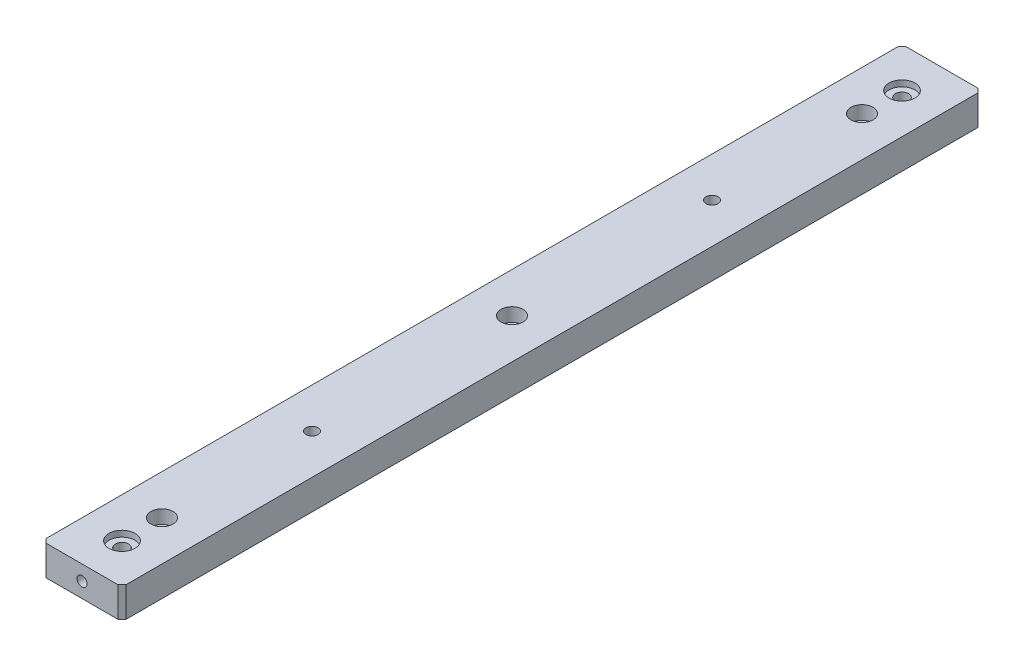
from build123d import *

# Parameters (mm, degrees)
SKETCH1_W                                    = 40
SKETCH1_H                                    = 430
BOSS_EXTRUDE1_DEPTH                          = 7.5
SKETCH2_R                                    = 6.5
CUT_EXTRUDE1_DEPTH                           = 3
HEX_SOCKET_CAP_SCREW_HOLE_TYPE_1_D           = 6.6
HEX_SOCKET_CAP_SCREW_HOLE_TYPE_1_CBORE_D     = 11
HEX_SOCKET_CAP_SCREW_HOLE_TYPE_1_CBORE_DEPTH = 6.8
M5_TAPPED_HOLE1_D                            = 4.2
M5_TAPPED_HOLE1_DEPTH                        = 15
M5_TAPPED_HOLE1_TIP                          = 1.2618073
CHAMFER1_SIZE                                = 2
HEX_SOCKET_CAP_SCREW_HOLE_TYPE_2_D           = 6.6
HEX_SOCKET_CAP_SCREW_HOLE_TYPE_2_CBORE_D     = 11
HEX_SOCKET_CAP_SCREW_HOLE_TYPE_2_CBORE_DEPTH = 6.8
M6_TAPPED_HOLE1_D                            = 5
M6_TAPPED_HOLE1_DEPTH                        = 13
M6_TAPPED_HOLE1_TIP                          = 1.502151548
M6_TAPPED_HOLE2_D                            = 5
M6_TAPPED_HOLE2_DEPTH                        = 13
M6_TAPPED_HOLE2_TIP                          = 1.502151548
F_6_0_6_DIAMETER_HOLE1_D                     = 6
F_6_0_6_DIAMETER_HOLE1_DEPTH                 = 17
F_6_0_6_DIAMETER_HOLE1_TIP                   = 1.802581857


with BuildPart() as part:
    # Sketch1 → Boss-Extrude1 (new, symmetric)
    with BuildSketch(Plane(origin=(0, 0, 0), x_dir=(1, 0, 0), z_dir=(0, 1, 0))):
        Rectangle(SKETCH1_W, SKETCH1_H)
    extrude(amount=BOSS_EXTRUDE1_DEPTH, both=True)

    # Sketch2 → Cut-Extrude1 (cut)
    with BuildSketch(Plane(origin=(0, 7.5, 0), x_dir=(1, 0, 0), z_dir=(0, 1, 0))):
        with Locations(Location((0, 195, 0), (0, 0, 270))):
            Circle(SKETCH2_R)
        with Locations(Location((0, -195, 0), (0, 0, 90))):
            Circle(SKETCH2_R)
    extrude(amount=-CUT_EXTRUDE1_DEPTH, mode=Mode.SUBTRACT)

    # Hex socket cap screw hole type 1 (through all)
    with Locations(Plane(origin=(0, -7.5, 0), x_dir=(-1, 0, 0), z_dir=(0, -1, 0))):
        with Locations((0, -195), (0, 195)):
            CounterBoreHole(HEX_SOCKET_CAP_SCREW_HOLE_TYPE_1_D / 2, HEX_SOCKET_CAP_SCREW_HOLE_TYPE_1_CBORE_D / 2, HEX_SOCKET_CAP_SCREW_HOLE_TYPE_1_CBORE_DEPTH)

    # M5 Tapped Hole1
    with Locations(Plane.ZY.offset(20)):
        with Locations((-195, 0), (195, 0), (-65, 0), (65, 0)):
            Hole(M5_TAPPED_HOLE1_D / 2, depth=M5_TAPPED_HOLE1_DEPTH)
            with Locations((0, 0, -(M5_TAPPED_HOLE1_DEPTH + M5_TAPPED_HOLE1_TIP / 2))):  # 118° drill point
                Cone(0, M5_TAPPED_HOLE1_D / 2, M5_TAPPED_HOLE1_TIP, mode=Mode.SUBTRACT)

    # Chamfer1
    chamfer1_edges = [part.edges().sort_by_distance(p)[0] for p in [
        (-20, 0, -215),
        (20, 0, -215),
        (20, 0, 215),
        (-20, 0, 215),
    ]]
    chamfer(chamfer1_edges, length=CHAMFER1_SIZE)

    # Hex socket cap screw hole type 2 (through all)
    with Locations(Plane(origin=(0, 7.5, 0), x_dir=(1, 0, 0), z_dir=(0, 1, 0))):
        with Locations((0, 175), (0, -175), (0, 0)):
            CounterBoreHole(HEX_SOCKET_CAP_SCREW_HOLE_TYPE_2_D / 2, HEX_SOCKET_CAP_SCREW_HOLE_TYPE_2_CBORE_D / 2, HEX_SOCKET_CAP_SCREW_HOLE_TYPE_2_CBORE_DEPTH)

    # M6 Tapped Hole1
    with Locations(Plane.XY.offset(215)):
        with Locations((0, 0)):
            Hole(M6_TAPPED_HOLE1_D / 2, depth=M6_TAPPED_HOLE1_DEPTH)
            with Locations((0, 0, -(M6_TAPPED_HOLE1_DEPTH + M6_TAPPED_HOLE1_TIP / 2))):  # 118° drill point
                Cone(0, M6_TAPPED_HOLE1_D / 2, M6_TAPPED_HOLE1_TIP, mode=Mode.SUBTRACT)

    # M6 Tapped Hole2
    with Locations(Plane(origin=(0, 0, -215), x_dir=(-1, 0, 0), z_dir=(0, 0, -1))):
        with Locations((0, 0)):
            Hole(M6_TAPPED_HOLE2_D / 2, depth=M6_TAPPED_HOLE2_DEPTH)
            with Locations((0, 0, -(M6_TAPPED_HOLE2_DEPTH + M6_TAPPED_HOLE2_TIP / 2))):  # 118° drill point
                Cone(0, M6_TAPPED_HOLE2_D / 2, M6_TAPPED_HOLE2_TIP, mode=Mode.SUBTRACT)

    # Ø6.0 (6) Diameter Hole1
    with Locations(Plane(origin=(0, -7.5, 0), x_dir=(-1, 0, 0), z_dir=(0, -1, 0))):
        with Locations((0, 100), (0, -100)):
            Hole(F_6_0_6_DIAMETER_HOLE1_D / 2, depth=F_6_0_6_DIAMETER_HOLE1_DEPTH)
            with Locations((0, 0, -(F_6_0_6_DIAMETER_HOLE1_DEPTH + F_6_0_6_DIAMETER_HOLE1_TIP / 2))):  # 118° drill point
                Cone(0, F_6_0_6_DIAMETER_HOLE1_D / 2, F_6_0_6_DIAMETER_HOLE1_TIP, mode=Mode.SUBTRACT)


solid = part.part
